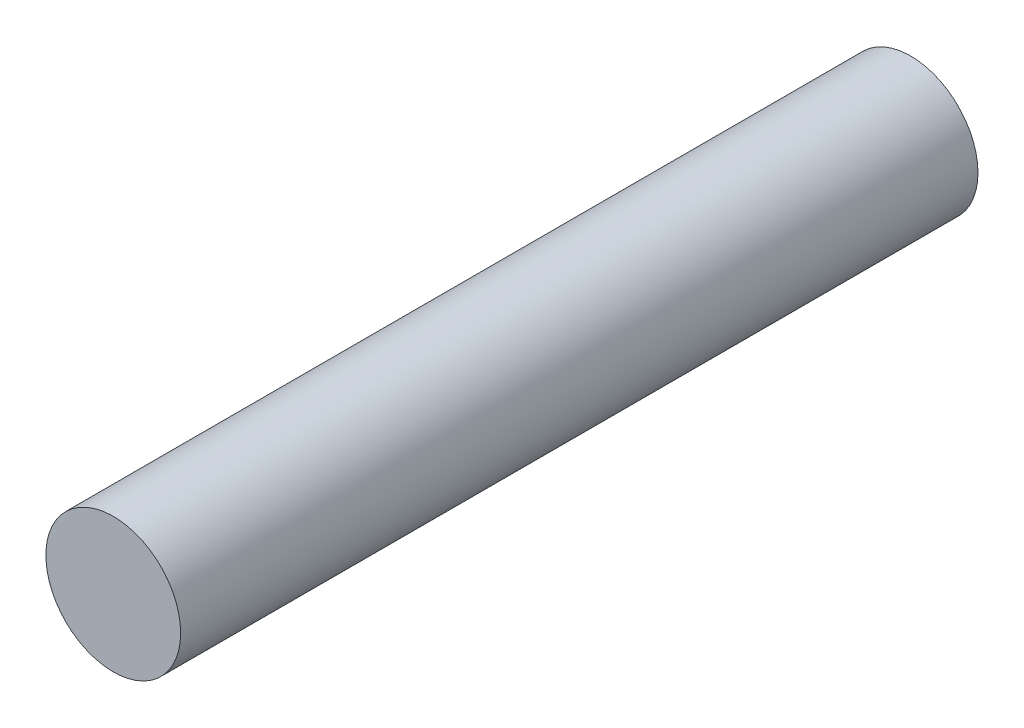
SolidWorks part; units mm, degrees
ref_plane "前视基准面" through (0, 0, 0) normal (0, 0, 1) x (1, 0, 0)
ref_plane "上视基准面" through (0, 0, 0) normal (0, 1, 0) x (1, 0, 0)
ref_plane "右视基准面" through (0, 0, 0) normal (1, 0, 0) x (0, 0, -1)
sketch "草图1" plane through (0, 0, 0) normal (0, 0, 1) x (1, 0, 0)
  circle A0 centre (0, 0) radius 6
  dimension "D1" = 12
extrude "凸台-拉伸1" add sketch "草图1" along normal mid plane 71
